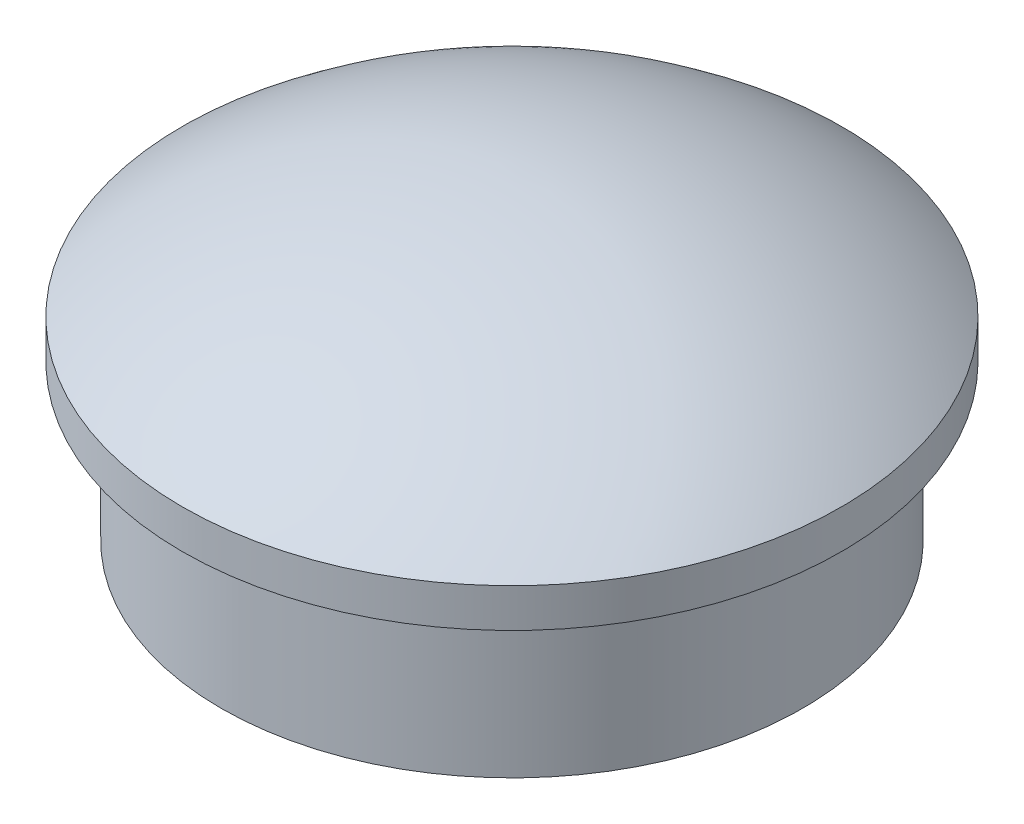
from build123d import *

# Parameters (mm, degrees)
SKETCH1_R           = 7.5
BOSS_EXTRUDE1_DEPTH = 4
SKETCH2_R           = 8.5
BOSS_EXTRUDE2_DEPTH = 1
DOME1_FACE_RADIUS   = 8.5
DOME1_HEIGHT        = 3
SKETCH3_R           = 6
CUT_EXTRUDE1_DEPTH  = 4
SCALE1_SCALE        = 0.5


with BuildPart() as part:
    # Sketch1 → Boss-Extrude1 (new body)
    with BuildSketch(Plane(origin=(0, 0, 0), x_dir=(1, 0, 0), z_dir=(0, 1, 0))):
        with Locations(Location((0, 0, 0), (0, 0, 270))):
            Circle(SKETCH1_R)
    extrude(amount=BOSS_EXTRUDE1_DEPTH)

    # Sketch2 → Boss-Extrude2 (add)
    with BuildSketch(Plane(origin=(0, 4, 0), x_dir=(1, 0, 0), z_dir=(0, 1, 0))):
        with Locations(Location((0, 0, 0), (0, 0, 270))):
            Circle(SKETCH2_R)
    extrude(amount=BOSS_EXTRUDE2_DEPTH)

    # Dome1: a dome of height H over a round flat face of radius A is a cap of a sphere of radius (A * A + H * H) / (2 * H)
    dome1_r = (DOME1_FACE_RADIUS * DOME1_FACE_RADIUS + DOME1_HEIGHT * DOME1_HEIGHT) / (2 * DOME1_HEIGHT)
    dome1_base = Plane((0, 5, 0), z_dir=(0, 1, 0))
    with Locations(dome1_base.offset(DOME1_HEIGHT - dome1_r)):
        dome1_ball = Sphere(dome1_r, mode=Mode.PRIVATE)
    add(split(dome1_ball, bisect_by=dome1_base, keep=Keep.TOP, mode=Mode.PRIVATE))

    # Sketch3 → Cut-Extrude1 (cut)
    with BuildSketch(Plane.XZ):
        with Locations(Location((0, 0, 0), (0, 0, 270))):
            Circle(SKETCH3_R)
    extrude(amount=-CUT_EXTRUDE1_DEPTH, mode=Mode.SUBTRACT)


with BuildPart() as part_1:
    # Scale1: scaled about (0, 4.383748239, 0)
    add(part.part.scale(SCALE1_SCALE).moved(Location((0, 2.191874119, 0))))


solid = part_1.part
